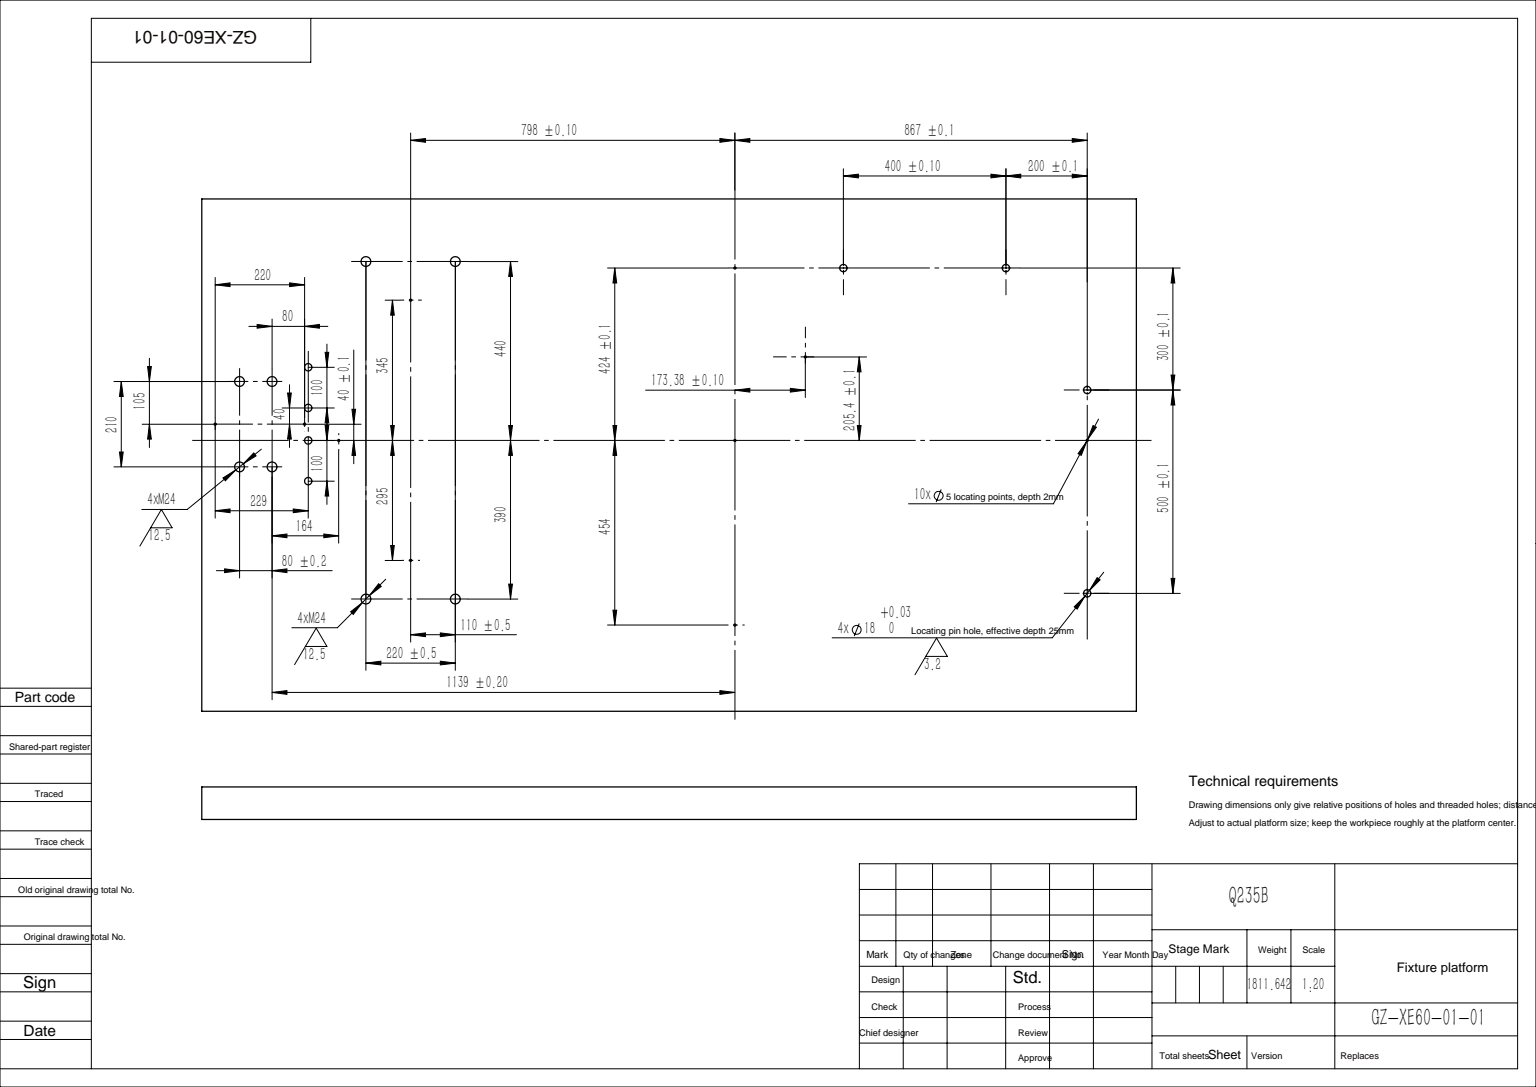
from build123d import *

# Parameters (mm, degrees)
SKETCH1_W           = 2300
SKETCH1_H           = 1260
SKETCH1_R           = 9
SKETCH1_R_2         = 12
SKETCH1_R_3         = 2.5
BOSS_EXTRUDE1_DEPTH = 80


with BuildPart() as part:
    # Sketch1 → Boss-Extrude1 (new body)
    with BuildSketch(Plane.XY):
        with Locations((1150, 630)):
            Rectangle(SKETCH1_W, SKETCH1_H)
        with Locations((1579, 1090)):
            Circle(SKETCH1_R, mode=Mode.SUBTRACT)
        with Locations((1979, 1090)):
            Circle(SKETCH1_R, mode=Mode.SUBTRACT)
        with Locations((2179, 790)):
            Circle(SKETCH1_R, mode=Mode.SUBTRACT)
        with Locations((2179, 290)):
            Circle(SKETCH1_R, mode=Mode.SUBTRACT)
        with Locations((93, 811)):
            Circle(SKETCH1_R_2, mode=Mode.SUBTRACT)
        with Locations((173, 811)):
            Circle(SKETCH1_R_2, mode=Mode.SUBTRACT)
        with Locations((93, 601)):
            Circle(SKETCH1_R_2, mode=Mode.SUBTRACT)
        with Locations((173, 601)):
            Circle(SKETCH1_R_2, mode=Mode.SUBTRACT)
        with Locations((404, 1106)):
            Circle(SKETCH1_R_2, mode=Mode.SUBTRACT)
        with Locations((624, 1106)):
            Circle(SKETCH1_R_2, mode=Mode.SUBTRACT)
        with Locations((404, 276)):
            Circle(SKETCH1_R_2, mode=Mode.SUBTRACT)
        with Locations((624, 276)):
            Circle(SKETCH1_R_2, mode=Mode.SUBTRACT)
        with Locations((2179, 666)):
            Circle(SKETCH1_R_3, mode=Mode.SUBTRACT)
        with Locations((337, 666)):
            Circle(SKETCH1_R_3, mode=Mode.SUBTRACT)
        with Locations((1312, 666)):
            Circle(SKETCH1_R_3, mode=Mode.SUBTRACT)
        with Locations((1485.38, 871.4)):
            Circle(SKETCH1_R_3, mode=Mode.SUBTRACT)
        with Locations((1312, 1090)):
            Circle(SKETCH1_R_3, mode=Mode.SUBTRACT)
        with Locations((1312, 212)):
            Circle(SKETCH1_R_3, mode=Mode.SUBTRACT)
        with Locations((514, 371)):
            Circle(SKETCH1_R_3, mode=Mode.SUBTRACT)
        with Locations((514, 1011)):
            Circle(SKETCH1_R_3, mode=Mode.SUBTRACT)
        with Locations((253, 706)):
            Circle(SKETCH1_R_3, mode=Mode.SUBTRACT)
        with Locations((33, 706)):
            Circle(SKETCH1_R_3, mode=Mode.SUBTRACT)
        with Locations((262, 746)):
            Circle(SKETCH1_R, mode=Mode.SUBTRACT)
        with Locations((262, 846)):
            Circle(SKETCH1_R, mode=Mode.SUBTRACT)
        with Locations((262, 666)):
            Circle(SKETCH1_R, mode=Mode.SUBTRACT)
        with Locations((262, 566)):
            Circle(SKETCH1_R, mode=Mode.SUBTRACT)
    extrude(amount=BOSS_EXTRUDE1_DEPTH)


solid = part.part
